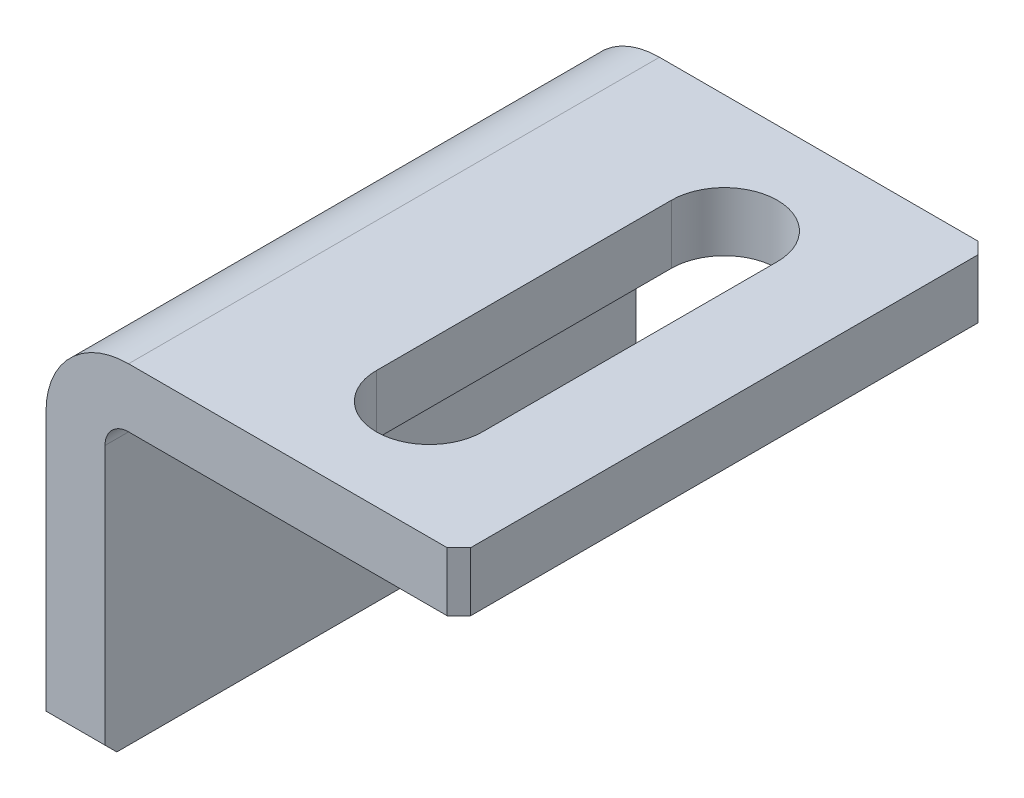
SolidWorks part; units mm, degrees
ref_plane "前视" through (0, 0, 0) normal (0, 0, 1) x (1, 0, 0)
ref_plane "上视" through (0, 0, 0) normal (0, 1, 0) x (1, 0, 0)
ref_plane "右视" through (0, 0, 0) normal (1, 0, 0) x (0, 0, -1)
sketch "草图1" plane through (0, 0, 0) normal (0, 0, 1) x (1, 0, 0)
  line L0 (0, 0) -> (0, 30)
  line L1 (0, 30) -> (35, 30)
  dimension "D1" = 30
  dimension "D2" = 35
extrude "拉伸-薄壁1" add sketch "草图1" along normal blind 45 thin
sketch "草图2" plane through (0, 25, 0) normal (0, -1, 0) x (1, 0, 0)
  line L0 (22.5, 35) -> (22.5, 10) construction
  line L1 (27, 35) -> (27, 10)
  line L2 (18, 35) -> (18, 10)
  line L3 (22.5, 22.5) -> (35, 22.5) construction
  line L4 (35, 45) -> (35, 0) construction
  arc A0 (27, 35) -> (18, 35) centre (22.5, 35) ccw
  arc A1 (18, 10) -> (27, 10) centre (22.5, 10) ccw
  point P2 (22.5, 22.5)
  dimension "D1" = 12.5
  dimension "D2" = 25
  dimension "D3" = 9
extrude "切除-拉伸1" cut sketch "草图2" against normal through all
fillet "圆角1" radius 2 1 edges at (5, 25, 22.5)
fillet "圆角2" radius 7 1 edges at (0, 30, 22.5)
chamfer "倒角1" distance 1 angle 45 4 edges at (2.5, 0, 0) (2.5, 0, 45) (35, 27.5, 0) (35, 27.5, 45)
